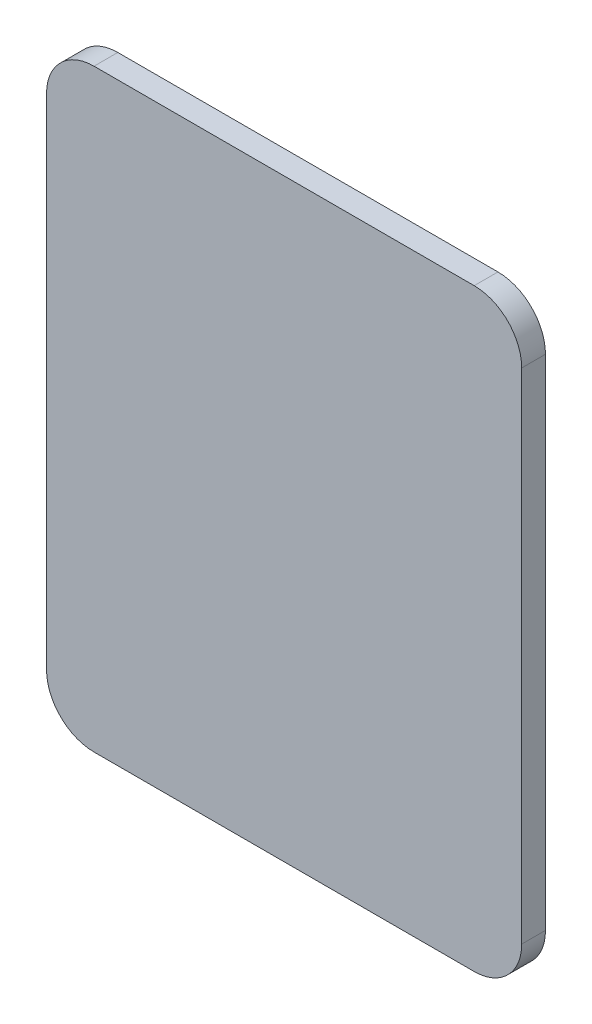
SolidWorks part; units mm, degrees
ref_plane "前视基准面" through (0, 0, 0) normal (0, 0, 1) x (1, 0, 0)
ref_plane "上视基准面" through (0, 0, 0) normal (0, 1, 0) x (1, 0, 0)
ref_plane "右视基准面" through (0, 0, 0) normal (1, 0, 0) x (0, 0, -1)
sketch "草图1" plane through (0, 0, 0) normal (0, 0, 1) x (1, 0, 0)
  line L1 (100, -125) -> (-100, -125)
  line L2 (100, -125) -> (100, 125)
  line L3 (100, 125) -> (-100, 125)
  line L4 (-100, -125) -> (-100, 125)
  line L5 (100, -125) -> (-100, 125) construction
  line L6 (100, 125) -> (-100, -125) construction
  point P0 (0, 0)
  dimension "D1" = 250
  dimension "D2" = 200
extrude "凸台-拉伸1" add sketch "草图1" along normal blind 10
fillet "圆角1" radius 20 4 edges at (-100, 125, 5) (-100, -125, 5) (100, -125, 5) (100, 125, 5)
hole_wizard "M8 螺纹孔2" positions "草图5" profile "草图4" tap size "M8" standard "GB"
sketch "草图5" plane through (0, 0, 0) normal (0, 0, -1) x (-1, 0, 0)
  point P0 (25, -100)
  point P3 (25, -65)
  point P6 (-25, -65)
  point P9 (-25, -100)
  point P12 (25, 100)
  point P15 (25, 65)
  point P18 (-25, 65)
  point P21 (-25, 100)
sketch "草图4" plane through (-25, -100, 0) normal (1, 0, 0) x (0, 1, 0)
  line L0 (0, 0) -> (0, 5)
  line L1 (0, 5) -> (3.4, 2.9571)
  line L2 (3.4, 2.9571) -> (3.4, 0.625)
  line L3 (3.4, 0.625) -> (4.025, 0)
  line L5 (4.025, 0) -> (0, 0)
  line L6 (-3.4, 0.625) -> (-4.025, 0) construction
  line L10 (0, 5) -> (-3.4, 2.9571) construction
  line L11 (0, -6.35) -> (0, 107.95) construction
  dimension "螺纹孔钻头直径" = 6.8
  dimension "螺纹孔钻头深度" = 5
  dimension "近端锥形沉头孔直径" = 8.05
  dimension "近端锥形沉头孔角度" = 90
  dimension "导头角度" = 118
cosmetic thread "孔螺蚊线1" parameters "D1"=16, "D2"=8
cosmetic thread "孔螺蚊线2" parameters "D1"=16, "D2"=8
cosmetic thread "孔螺蚊线3" parameters "D1"=16, "D2"=8
cosmetic thread "孔螺蚊线4" parameters "D1"=16, "D2"=8
cosmetic thread "孔螺蚊线5" parameters "D1"=16, "D2"=8
cosmetic thread "孔螺蚊线6" parameters "D1"=16, "D2"=8
cosmetic thread "孔螺蚊线7" parameters "D1"=16, "D2"=8
cosmetic thread "孔螺蚊线8" parameters "D1"=16, "D2"=8
hole_wizard "M6 螺纹孔1" positions "草图6" profile "草图7" tap size "M6" standard "GB"
sketch "草图6" plane through (0, 0, 0) normal (0, 0, -1) x (-1, 0, 0)
  point P0 (70, 20)
  point P3 (30, 20)
  point P6 (70, -20)
  point P9 (30, -20)
  point P12 (-30, 20)
  point P15 (-30, -20)
  point P18 (-70, 20)
  point P21 (-70, -20)
sketch "草图7" plane through (-70, 20, 0) normal (1, 0, 0) x (0, 1, 0)
  line L0 (0, 0) -> (0, 8)
  line L1 (0, 8) -> (2.5, 6.4978)
  line L2 (2.5, 6.4978) -> (2.5, 0.525)
  line L3 (2.5, 0.525) -> (3.025, 0)
  line L5 (3.025, 0) -> (0, 0)
  line L6 (-2.5, 0.525) -> (-3.025, 0) construction
  line L10 (0, 8) -> (-2.5, 6.4978) construction
  line L11 (0, -6.35) -> (0, 107.95) construction
  dimension "螺纹孔钻头直径" = 5
  dimension "螺纹孔钻头深度" = 8
  dimension "近端锥形沉头孔直径" = 6.05
  dimension "近端锥形沉头孔角度" = 90
  dimension "导头角度" = 118
cosmetic thread "孔螺蚊线9" parameters "D1"=12, "D2"=6
cosmetic thread "孔螺蚊线10" parameters "D1"=12, "D2"=6
cosmetic thread "孔螺蚊线11" parameters "D1"=12, "D2"=6
cosmetic thread "孔螺蚊线12" parameters "D1"=12, "D2"=6
cosmetic thread "孔螺蚊线13" parameters "D1"=12, "D2"=6
cosmetic thread "孔螺蚊线14" parameters "D1"=12, "D2"=6
cosmetic thread "孔螺蚊线15" parameters "D1"=12, "D2"=6
cosmetic thread "孔螺蚊线16" parameters "D1"=12, "D2"=6
